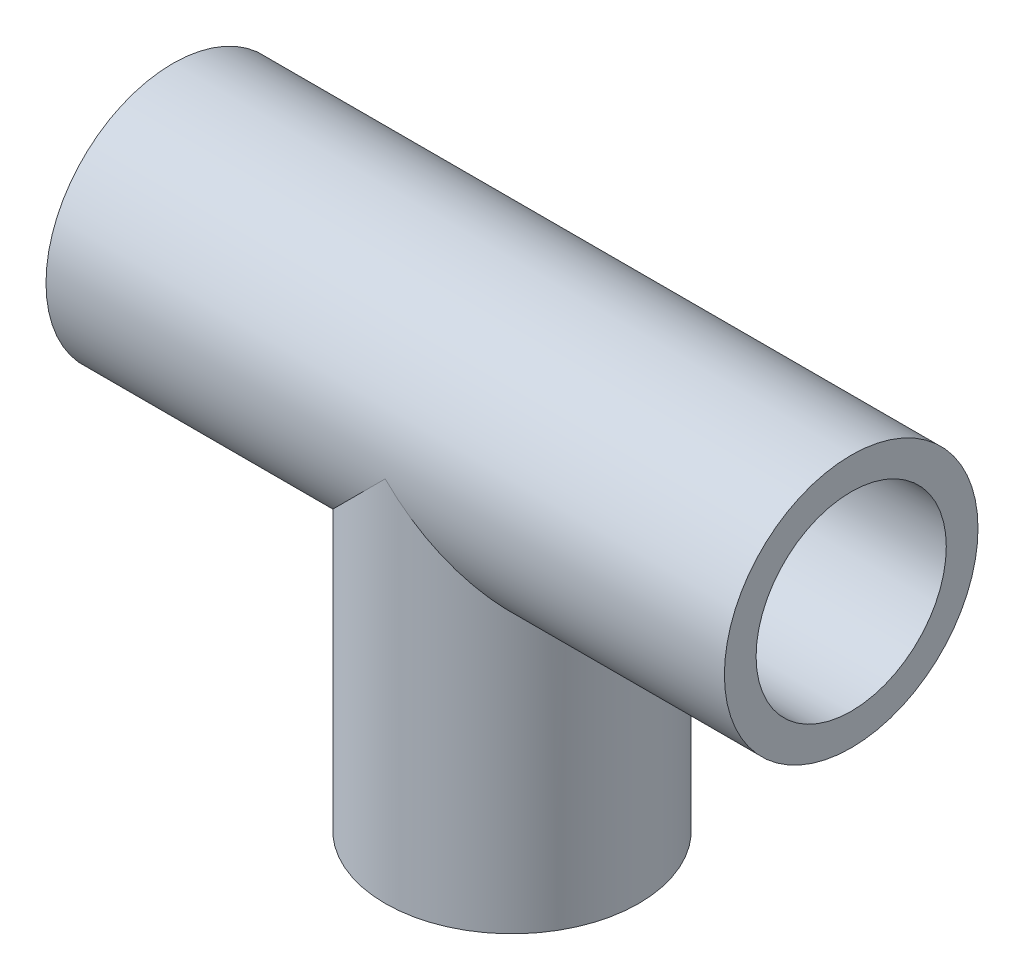
from build123d import *

# Parameters (mm, degrees)
SWEEP_THIN_PART_1_PROFILE_R   = 10
SWEEP_THIN_PART_1_PROFILE_R_2 = 7.5
SWEEP_THIN_PART_2_PROFILE_R   = 10
SWEEP_THIN_PART_2_PROFILE_R_2 = 7.5
SKETCH15_R                    = 7.5
CUT_EXTRUDE1_DEPTH            = 62.67049551
SKETCH18_R                    = 7.5
CUT_EXTRUDE2_DEPTH            = 30


with BuildPart() as part:
    # Sweep-thin part 1: sweep along a path in Sketch1
    with BuildLine(Plane.XY) as sweep_thin_part_1_path:
        Line((-26.75, 0), (26.75, 0))
    # Sweep-thin part 1 profile (on start of the path) → Sweep-thin part 1 (sweep)
    with BuildSketch(Plane.YZ.offset(-26.75)):
        Circle(SWEEP_THIN_PART_1_PROFILE_R)
        Circle(SWEEP_THIN_PART_1_PROFILE_R_2, mode=Mode.SUBTRACT)
    sweep(path=sweep_thin_part_1_path.line)

    # Sweep-thin part 2: sweep along a path in Sketch8
    with BuildLine(Plane.XY) as sweep_thin_part_2_path:
        Line((0, 0), (0, -29))
    # Sweep-thin part 2 profile (on start of the path) → Sweep-thin part 2 (sweep)
    with BuildSketch(Plane(origin=(0, 0, 0), x_dir=(-1, 0, 0), z_dir=(0, -1, 0))):
        Circle(SWEEP_THIN_PART_2_PROFILE_R)
        Circle(SWEEP_THIN_PART_2_PROFILE_R_2, mode=Mode.SUBTRACT)
    sweep(path=sweep_thin_part_2_path.line)

    # Sketch15 → Cut-Extrude1 (cut, through all)
    with BuildSketch(Plane.ZY.offset(26.75)):
        with Locations(Location((0, 0, 0), (0, 0, 90))):
            Circle(SKETCH15_R)
    extrude(amount=-CUT_EXTRUDE1_DEPTH, mode=Mode.SUBTRACT)

    # Sketch18 → Cut-Extrude2 (cut)
    with BuildSketch(Plane.XZ.offset(29)):
        Circle(SKETCH18_R)
    extrude(amount=-CUT_EXTRUDE2_DEPTH, mode=Mode.SUBTRACT)


solid = part.part
